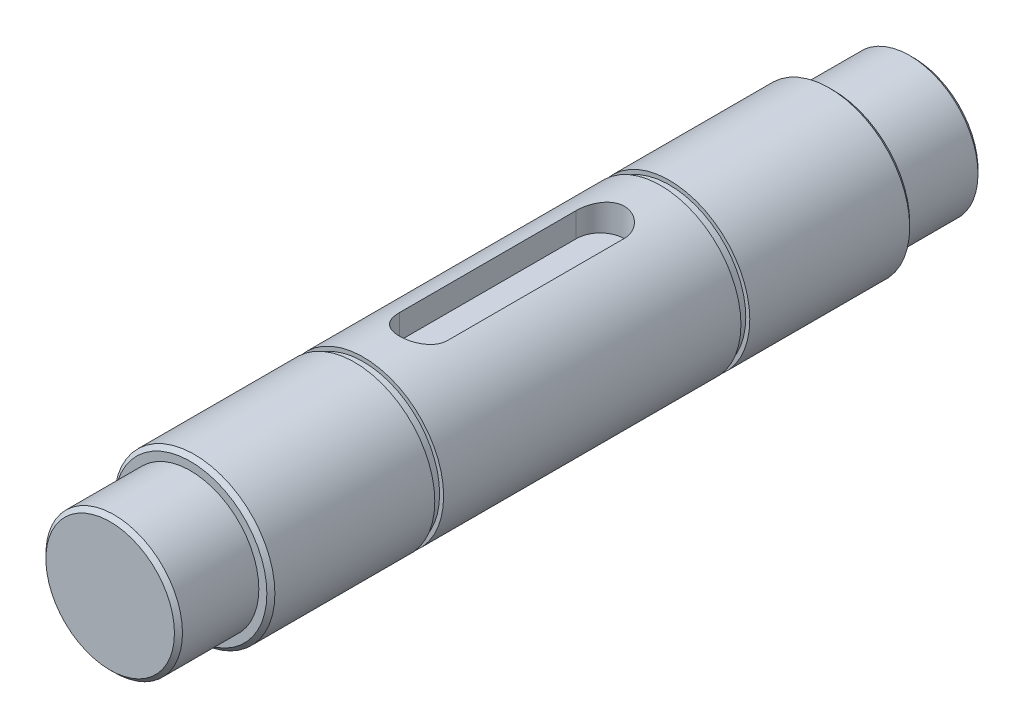
SolidWorks part; units mm, degrees
ref_plane "前视" through (0, 0, 0) normal (0, 0, 1) x (1, 0, 0)
ref_plane "上视" through (0, 0, 0) normal (0, 1, 0) x (1, 0, 0)
ref_plane "右视" through (0, 0, 0) normal (1, 0, 0) x (0, 0, -1)
sketch "草图1" plane through (0, 0, 0) normal (0, 0, 1) x (1, 0, 0)
  circle A0 centre (0, 0) radius 10
  dimension "D1" = 20
extrude "凸台-拉伸1" add sketch "草图1" along normal mid plane 80
sketch "草图2" plane through (0, 0, 40) normal (0, 0, 1) x (1, 0, 0)
  circle A0 centre (0, 0) radius 8.5
  dimension "D1" = 17
extrude "凸台-拉伸2" add sketch "草图2" along normal blind 10
ref_plane "基准面1" through (0, 0, 18.5) normal (0, 0, 1) x (1, 0, 0)
sketch "草图4" plane through (0, 0, 18.5) normal (0, 0, 1) x (1, 0, 0)
  circle A0 centre (0, 0) radius 10
  circle A1 centre (0, 0) radius 9.5
  dimension "D1" = 20
  dimension "D2" = 19
extrude "切除-拉伸1" cut sketch "草图4" along normal blind 1.1
mirror "镜向1" about plane through (0, 0, 0) normal (0, 0, 1) of "凸台-拉伸2", "切除-拉伸1"
chamfer "倒角1" distance 0.5 angle 45 4 edges at (10, 0, -40) (8.5, 0, -50) (10, 0, 40) (8.5, 0, 50)
ref_plane "基准面2" through (0, 10, 0) normal (0, 1, 0) x (1, 0, 0)
sketch "草图5" plane through (0, 10, 0) normal (0, 1, 0) x (1, 0, 0)
  line L0 (0, 11) -> (0, -11) construction
  line L1 (3, 11) -> (3, -11)
  line L2 (-3, 11) -> (-3, -11)
  arc A0 (3, 11) -> (-3, 11) centre (0, 11) ccw
  arc A1 (-3, -11) -> (3, -11) centre (0, -11) ccw
  point P3 (0, 0)
  dimension "D1" = 6
  dimension "D2" = 22
extrude "切除-拉伸2" cut sketch "草图5" against normal blind 3.5
